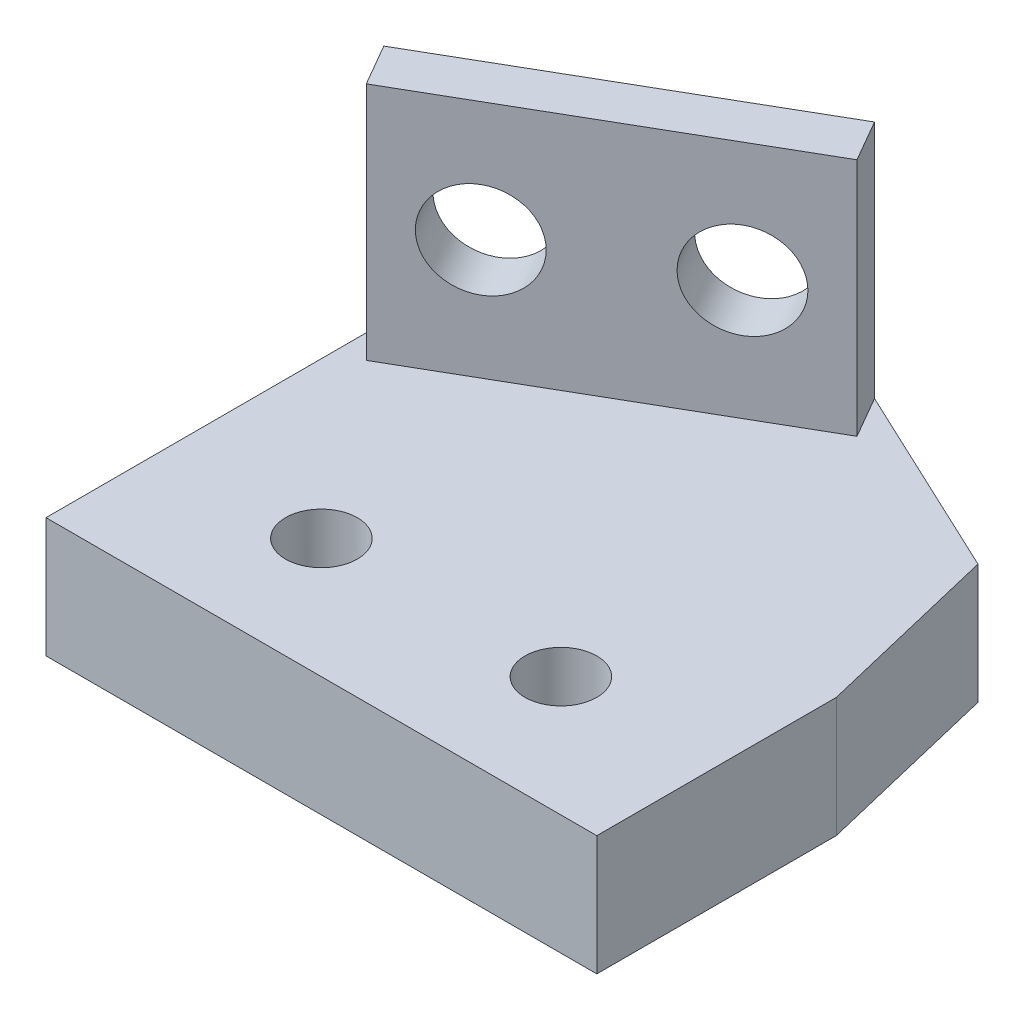
SolidWorks part; units mm, degrees
ref_plane "Front Plane" through (0, 0, 0) normal (0, 0, 1) x (1, 0, 0)
ref_plane "Top Plane" through (0, 0, 0) normal (0, 1, 0) x (1, 0, 0)
ref_plane "Right Plane" through (0, 0, 0) normal (1, 0, 0) x (0, 0, -1)
other "Configuration Table"
sketch "Sketch1" plane through (0, 0, 0) normal (0, 1, 0) x (1, 0, 0)
  line L0 (0, 0) -> (-23, 0)
  line L1 (-23, 0) -> (-23, 14.1057)
  line L2 (-23, 14.1057) -> (-10.0096, 21.6057)
  line L5 (0, 10) -> (0, 0)
  line L6 (-10.0096, 21.6057) -> (-1.8632, 17.78)
  line L7 (-1.8632, 17.78) -> (0, 10)
  dimension "D1" = 120
  dimension "D2" = 15
  dimension "D3" = 10
  dimension "D4" = 9
  dimension "D5" = 23
  dimension "D6" = 8
  dimension "D7" = 124.845
extrude "Boss-Extrude1" add sketch "Sketch1" along normal blind 5
sketch "Sketch2" plane through (0, 5, 0) normal (0, 1, 0) x (1, 0, 0)
  line L0 (-22, 12.3736) -> (-9.0096, 19.8736)
  line L1 (-23, 14.1057) -> (-23, 0) construction
  line L4 (-10.0096, 21.6057) -> (-23, 14.1057)
  line L5 (-10.0096, 21.6057) -> (-23, 14.1057) construction
  line L7 (-23, 14.1057) -> (-22, 12.3736)
  line L8 (-10.0096, 21.6057) -> (-9.0096, 19.8736)
  dimension "D1" = 2
extrude "Boss-Extrude2" add sketch "Sketch2" along normal blind 10
sketch "Sketch3" plane through (-10.8579, 0, -18.8065) normal (0.5, 0, 0.866) x (0.866, 0, -0.5)
  line L1 (-5.3657, 15) -> (-5.3657, 5) construction
  line L2 (-12.8657, 15) -> (2.1343, 15) construction
  line L3 (-12.8657, 5) -> (2.1343, 5) construction
  circle A0 centre (-9.3657, 10) radius 2
  circle A1 centre (-1.3657, 10) radius 2
  dimension "D1" = 4
  dimension "D2" = 4
  dimension "D3" = 8
  dimension "D4" = 4
  dimension "D5" = 5
extrude "Cut-Extrude1" cut sketch "Sketch3" against normal through all both and the other way through all
sketch "Sketch4" plane through (0, 5, 0) normal (0, 1, 0) x (1, 0, 0)
  line L0 (-23, 0) -> (0, 0) construction
  line L1 (-11.5, 0) -> (-11.5, 22.1273) construction
  circle A0 centre (-16.5, 5) radius 1.5
  circle A1 centre (-6.5, 5) radius 1.5
  dimension "D1" = 3
  dimension "D2" = 3
  dimension "D3" = 5
  dimension "D4" = 5
  dimension "D5" = 5
  dimension "D6" = 5
extrude "Cut-Extrude2" cut sketch "Sketch4" against normal through all both and the other way through all
